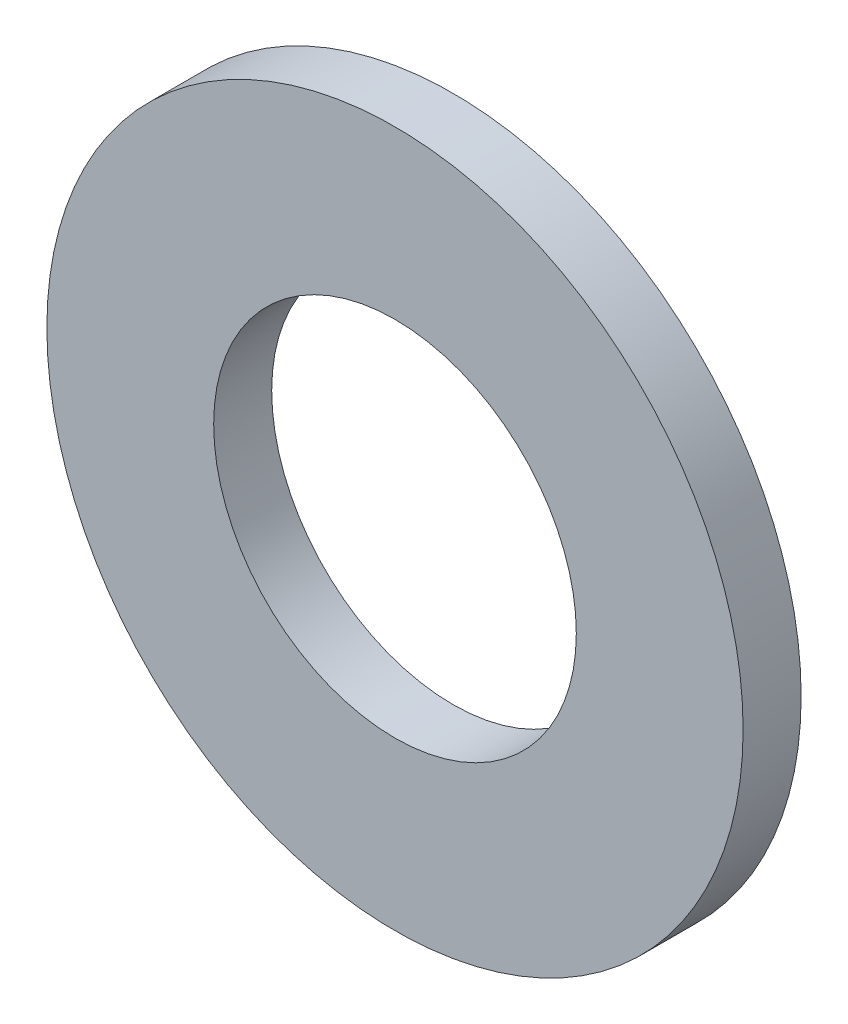
SolidWorks part; units mm, degrees
ref_plane "Front Plane" through (0, 0, 0) normal (0, 0, 1) x (1, 0, 0)
ref_plane "Top Plane" through (0, 0, 0) normal (0, 1, 0) x (1, 0, 0)
ref_plane "Right Plane" through (0, 0, 0) normal (1, 0, 0) x (0, 0, -1)
sketch "Sketch2" plane through (0, 0, 0) normal (0, 0, 1) x (1, 0, 0)
  circle A0 centre (0, 0) radius 6
  circle A1 centre (0, 0) radius 3.125
  dimension "D1" = 6.25
  dimension "D2" = 12
extrude "Boss-Extrude1" add sketch "Sketch2" along normal blind 1
